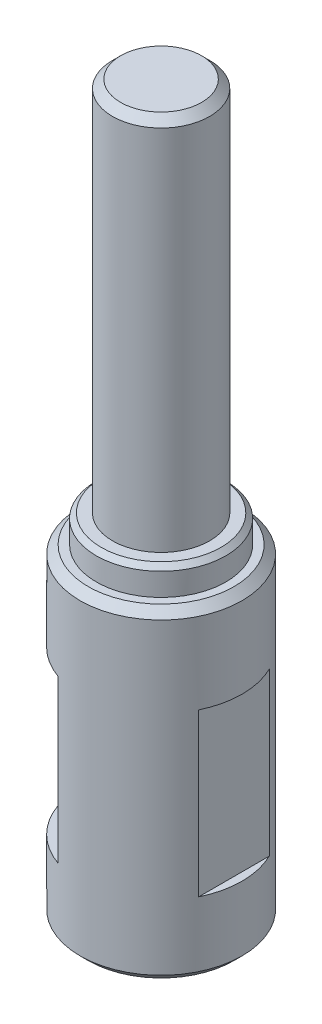
from build123d import *

# Parameters (mm, degrees)
SKETCH1_R           = 3
BOSS_EXTRUDE1_DEPTH = 20.5
SKETCH2_R           = 4
BOSS_EXTRUDE2_DEPTH = 1.2
SKETCH5_R           = 3
BOSS_EXTRUDE3_DEPTH = 23.2
CHAMFER3_SIZE       = 0.5
BOSS_EXTRUDE4_START = 20.5
SKETCH6_R           = 4
BOSS_EXTRUDE4_DEPTH = 20.5
CHAMFER4_SIZE       = 0.3
SKETCH9_R           = 5
BOSS_EXTRUDE5_DEPTH = 20
CHAMFER5_SIZE       = 0.5
SKETCH10_W          = 1
SKETCH10_H          = 10
CUT_EXTRUDE2_DEPTH  = 10
CIRPATTERN2_COUNT   = 2
CIRPATTERN2_ANGLE   = 135


with BuildPart() as part:
    # Sketch1 → Boss-Extrude1 (new body)
    with BuildSketch(Plane(origin=(0, 0, 0), x_dir=(1, 0, 0), z_dir=(0, 1, 0))):
        with Locations(Location((0, 0, 0), (0, 0, 270))):
            Circle(SKETCH1_R)
    extrude(amount=BOSS_EXTRUDE1_DEPTH)

    # Sketch2 → Boss-Extrude2 (add)
    with BuildSketch(Plane(origin=(0, 20.5, 0), x_dir=(1, 0, 0), z_dir=(0, 1, 0))):
        with Locations(Location((0, 0, 0), (0, 0, 270))):
            Circle(SKETCH2_R)
    extrude(amount=BOSS_EXTRUDE2_DEPTH)

    # Sketch5 → Boss-Extrude3 (add)
    with BuildSketch(Plane(origin=(0, 21.7, 0), x_dir=(1, 0, 0), z_dir=(0, 1, 0))):
        with Locations(Location((0, 0, 0), (0, 0, 270))):
            Circle(SKETCH5_R)
    extrude(amount=BOSS_EXTRUDE3_DEPTH)

    # Chamfer3
    chamfer3_edges = [part.edges().sort_by_distance(p)[0] for p in [
        (0, 44.9, -3),
    ]]
    chamfer(chamfer3_edges, length=CHAMFER3_SIZE)

    # Sketch6 → Boss-Extrude4 (add)
    with BuildSketch(Plane.XZ.offset(-20.5).offset(BOSS_EXTRUDE4_START)):
        with Locations(Location((0, 0, 0), (0, 0, 90))):
            Circle(SKETCH6_R)
    extrude(amount=-BOSS_EXTRUDE4_DEPTH)

    # Chamfer4
    chamfer4_edges = [part.edges().sort_by_distance(p)[0] for p in [
        (0, 21.7, -4),
    ]]
    chamfer(chamfer4_edges, length=CHAMFER4_SIZE)

    # Sketch9 → Boss-Extrude5 (add)
    with BuildSketch(Plane.XZ):
        with Locations(Location((0, 0, 0), (0, 0, 270))):
            Circle(SKETCH9_R)
    extrude(amount=-BOSS_EXTRUDE5_DEPTH)

    # Chamfer5
    chamfer5_edges = [part.edges().sort_by_distance(p)[0] for p in [
        (0, 0, 5),
        (0, 20, 5),
    ]]
    chamfer(chamfer5_edges, length=CHAMFER5_SIZE)

    # Sketch10 → Cut-Extrude2 (cut, symmetric)
    with BuildSketch(Plane.XY):
        with Locations((5, 9.5)):
            Rectangle(SKETCH10_W, SKETCH10_H)
    cut_extrude2 = extrude(amount=CUT_EXTRUDE2_DEPTH, both=True, mode=Mode.SUBTRACT)

    # CirPattern2: Cut-Extrude2 ×2 about axis
    cirpattern2_axis = Axis((0, 44.9, 0), (0, -1, 0))
    for i in range(1, CIRPATTERN2_COUNT):
        add(cut_extrude2.rotate(cirpattern2_axis, i * CIRPATTERN2_ANGLE / (CIRPATTERN2_COUNT - 1)), mode=Mode.SUBTRACT)


solid = part.part
